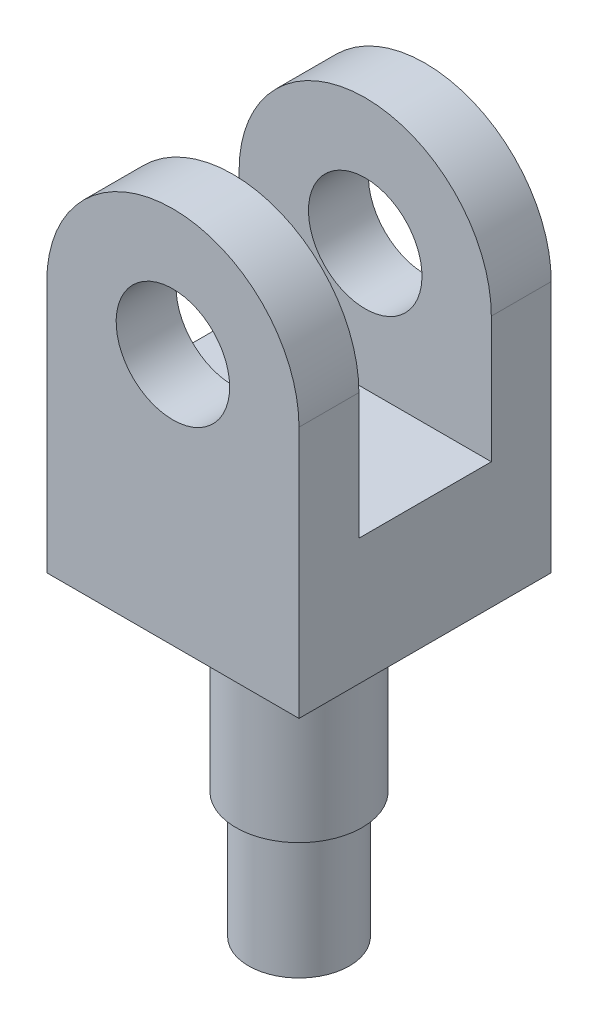
SolidWorks part; units mm, degrees
material "Q235B"
ref_plane "Front Plane" through (0, 0, 0) normal (0, 0, 1) x (1, 0, 0)
ref_plane "Top Plane" through (0, 0, 0) normal (0, 1, 0) x (1, 0, 0)
ref_plane "Right Plane" through (0, 0, 0) normal (1, 0, 0) x (0, 0, -1)
sketch "Sketch1" plane through (0, 0, 0) normal (0, 0, 1) x (1, 0, 0)
  line L1 (140.4025, -159.5975) -> (-59.5975, -159.5975)
  line L2 (140.4025, -159.5975) -> (140.4025, 40.4025)
  line L3 (140.4025, 40.4025) -> (-59.5975, 40.4025) construction
  line L4 (-59.5975, -159.5975) -> (-59.5975, 40.4025)
  line L5 (140.4025, -159.5975) -> (-59.5975, 40.4025) construction
  line L6 (140.4025, 40.4025) -> (-59.5975, -159.5975) construction
  arc A0 (140.4025, 40.4025) -> (-59.5975, 40.4025) centre (40.4025, 40.4025) ccw
  circle A1 centre (40.4025, 40.4025) radius 45
  point P0 (40.4025, -59.5975)
  dimension "D1" = 90
  dimension "D2" = 100
extrude "Boss-Extrude2" add sketch "Sketch1" along normal blind 200
sketch "Sketch2" plane through (140.4025, 0, 0) normal (1, 0, 0) x (0, 0, -1)
  line L0 (-100, 140.4025) -> (-100, -159.5975) construction
  line L1 (0, 140.4025) -> (-200, 140.4025) construction
  line L2 (-200, -159.5975) -> (0, -159.5975) construction
  line L4 (-152.5, 258.4524) -> (-47.5, 258.4524)
  line L5 (-152.5, 258.4524) -> (-152.5, -59.5975)
  line L6 (-152.5, -59.5975) -> (-47.5, -59.5975)
  line L7 (-47.5, 258.4524) -> (-47.5, -59.5975)
  line L8 (-152.5, 258.4524) -> (-47.5, -59.5975) construction
  line L9 (-152.5, -59.5975) -> (-47.5, 258.4524) construction
  point P6 (-100, 99.4274)
  dimension "D2" = 100
  dimension "D3" = 105
extrude "Cut-Extrude1" cut sketch "Sketch2" against normal through all
sketch "Sketch3" plane through (0, -159.5975, 0) normal (0, -1, 0) x (1, 0, 0)
  line L0 (40.4025, 200) -> (40.4025, 0) construction
  line L1 (-59.5975, 200) -> (140.4025, 200) construction
  line L2 (-59.5975, 0) -> (140.4025, 0) construction
  circle A0 centre (40.4025, 100) radius 50
  dimension "D1" = 100
extrude "Boss-Extrude3" add sketch "Sketch3" along normal blind 140
sketch "Sketch4" plane through (0, -299.5975, 0) normal (0, -1, 0) x (1, 0, 0)
  circle A0 centre (40.4025, 100) radius 50
  dimension "D1" = 100
extrude "Boss-Extrude4" add sketch "Sketch4" along normal blind 10
sketch "Sketch5" plane through (0, -309.5975, 0) normal (0, -1, 0) x (1, 0, 0)
  circle A0 centre (40.4025, 100) radius 40
  dimension "D1" = 80
extrude "Boss-Extrude5" add sketch "Sketch5" along normal blind 100
equation "\"dhgs\"= \"代号公式\""
equation "\"mcgs\"= \"名称公式\""
